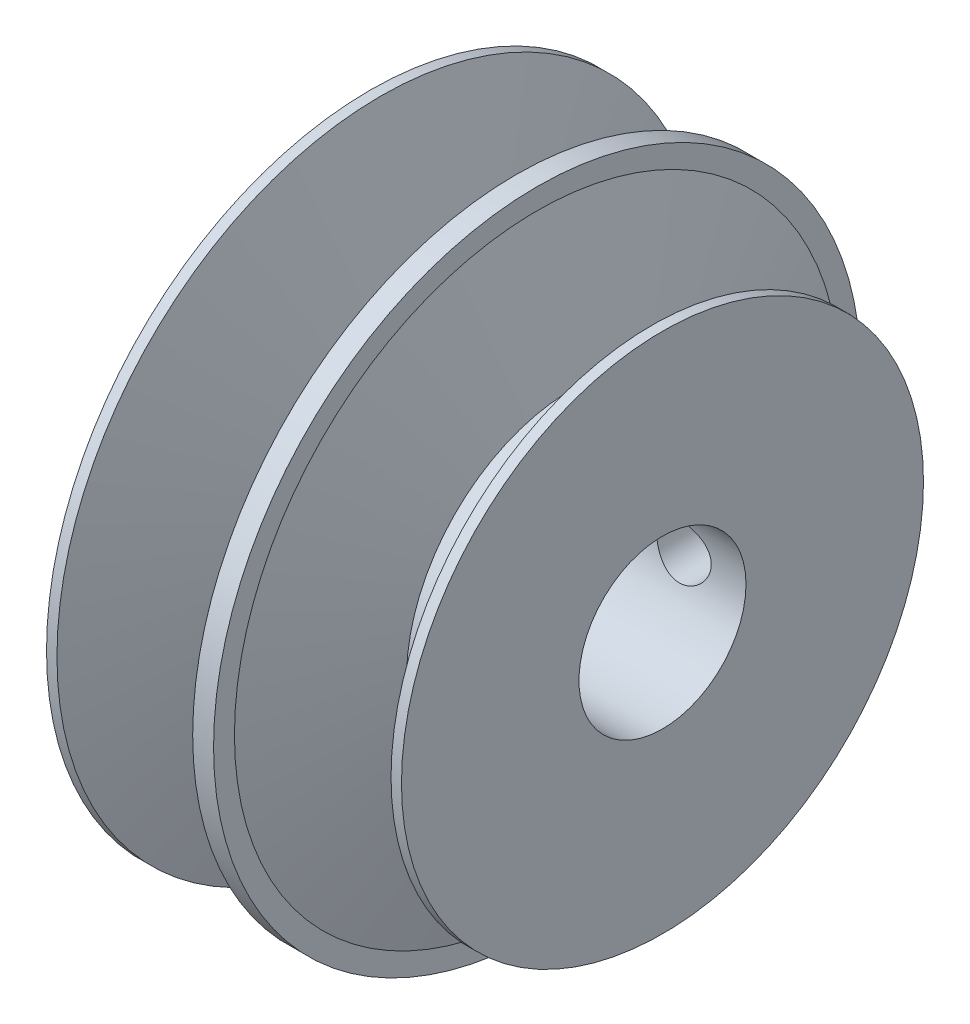
from build123d import *

# Parameters (mm, degrees)
SKETCH2_R           = 14.854735332
SKETCH2_R_2         = 8
BOSS_EXTRUDE1_DEPTH = 28
SKETCH3_R           = 14
CUT_EXTRUDE1_DEPTH  = 16
SKETCH6_W           = 2.60985
SKETCH6_H           = 47.082912009


with BuildPart() as part:
    # Sketch1 → Revolve1 (revolve)
    with BuildSketch(Plane.XY, mode=Mode.PRIVATE) as revolve1_sk:
        Polygon((-43.610341394, 31), (-42.610341394, 31), (-38.591103508, 16), (-33.62957928, 16), (-29.610341394, 31), (-27.610341394, 31), (-27.610341394, 29), (-24.127001892, 16), (-19.021884126, 16), (-16.610341394, 25), (-15.610341394, 25), (-15.610341394, 14), (-43.610341394, 14), align=None)
    revolve(revolve1_sk.sketch.rotate(Axis((-65.147183499, 0, 0), (1, 0, 0)), 90), axis=Axis((-65.147183499, 0, 0), (1, 0, 0)))

    # Sketch2 → Boss-Extrude1 (add, through all)
    with BuildSketch(Plane(origin=(-15.610341394, 0, 0), x_dir=(0, 0, -1), z_dir=(1, 0, 0))):
        Circle(SKETCH2_R)
        Circle(SKETCH2_R_2, mode=Mode.SUBTRACT)
    extrude(amount=-BOSS_EXTRUDE1_DEPTH)

    # Sketch3 → Cut-Extrude1 (cut)
    with BuildSketch(Plane.ZY.offset(43.610341394)):
        Circle(SKETCH3_R)
    extrude(amount=-CUT_EXTRUDE1_DEPTH, mode=Mode.SUBTRACT)

    # Sketch6 → #5 (0.2055) Diameter Hole1 (revolve, cut)
    with BuildSketch(Plane(origin=(-21.548066642, 0.042850676, 15.999942619), x_dir=(0, -0.9999964137036997, 0.0026781672351362563), z_dir=(1, 0, 0))):
        with Locations((1.304925, 23.541456005)):
            Rectangle(SKETCH6_W, SKETCH6_H)
    revolve(axis=Axis((-21.548066642, 0.059857038, 22.349919846), (0, -0.0026781672351362563, -0.9999964137036995)), mode=Mode.SUBTRACT)


solid = part.part
